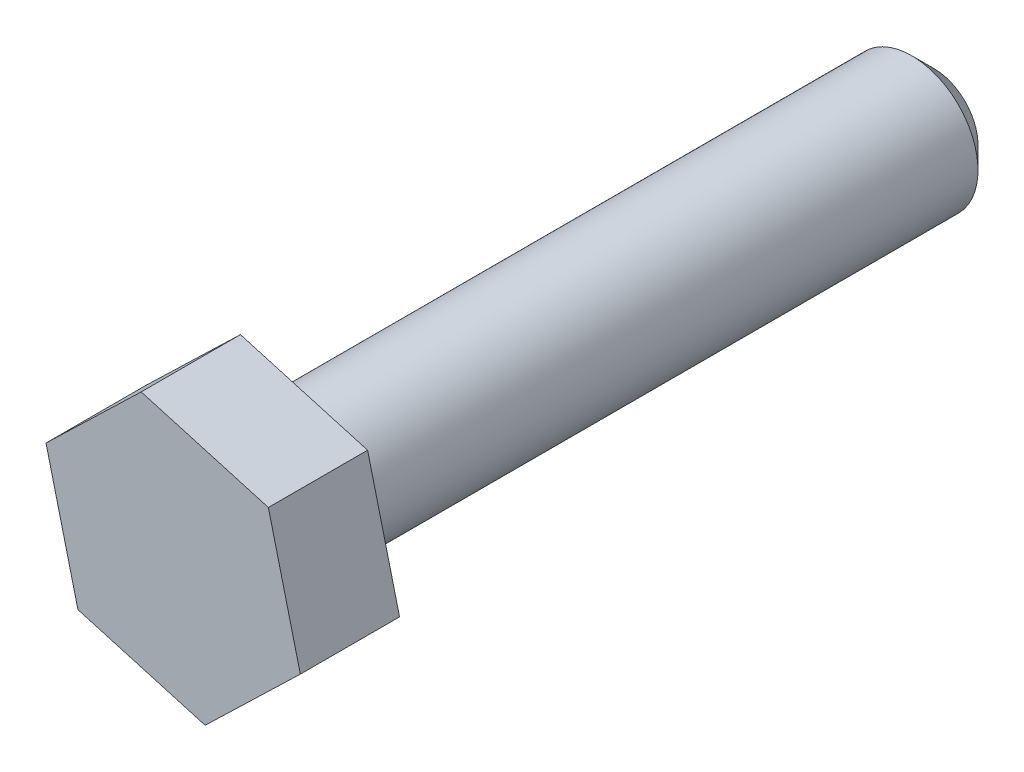
from build123d import *

# Parameters (mm, degrees)
SKETCH1_R           = 6
BOSS_EXTRUDE1_DEPTH = 4.5
SKETCH2_OUTSIDE_W   = 17.512
SKETCH2_OUTSIDE_H   = 17.512
CUT_EXTRUDE1_DEPTH  = 4.5
SKETCH3_R           = 3
BOSS_EXTRUDE2_DEPTH = 30
CHAMFER1_SIZE       = 1


with BuildPart() as part:
    # Sketch1 → Boss-Extrude1 (new body)
    with BuildSketch(Plane.XY):
        Circle(SKETCH1_R)
    extrude(amount=BOSS_EXTRUDE1_DEPTH)

    # Sketch2 outside → Cut-Extrude1 (cut)
    with BuildSketch(Plane(origin=(0, 0, 0), x_dir=(-1, 0, 0), z_dir=(0, 0, -1))):
        Rectangle(SKETCH2_OUTSIDE_W, SKETCH2_OUTSIDE_H)
        Polygon((4.317619028, -4.16631323), (5.766942611, 1.656011147), (1.449323583, 5.822324377), (-4.317619028, 4.16631323), (-5.766942611, -1.656011147), (-1.449323583, -5.822324377), align=None, mode=Mode.SUBTRACT)
    extrude(amount=-CUT_EXTRUDE1_DEPTH, mode=Mode.SUBTRACT)

    # Sketch3 → Boss-Extrude2 (add)
    with BuildSketch(Plane(origin=(0, 0, 0), x_dir=(-1, 0, 0), z_dir=(0, 0, -1))):
        Circle(SKETCH3_R)
    extrude(amount=BOSS_EXTRUDE2_DEPTH)

    # Chamfer1
    chamfer1_edges = [part.edges().sort_by_distance(p)[0] for p in [
        (3, 0, -30),
    ]]
    chamfer(chamfer1_edges, length=CHAMFER1_SIZE)


solid = part.part
